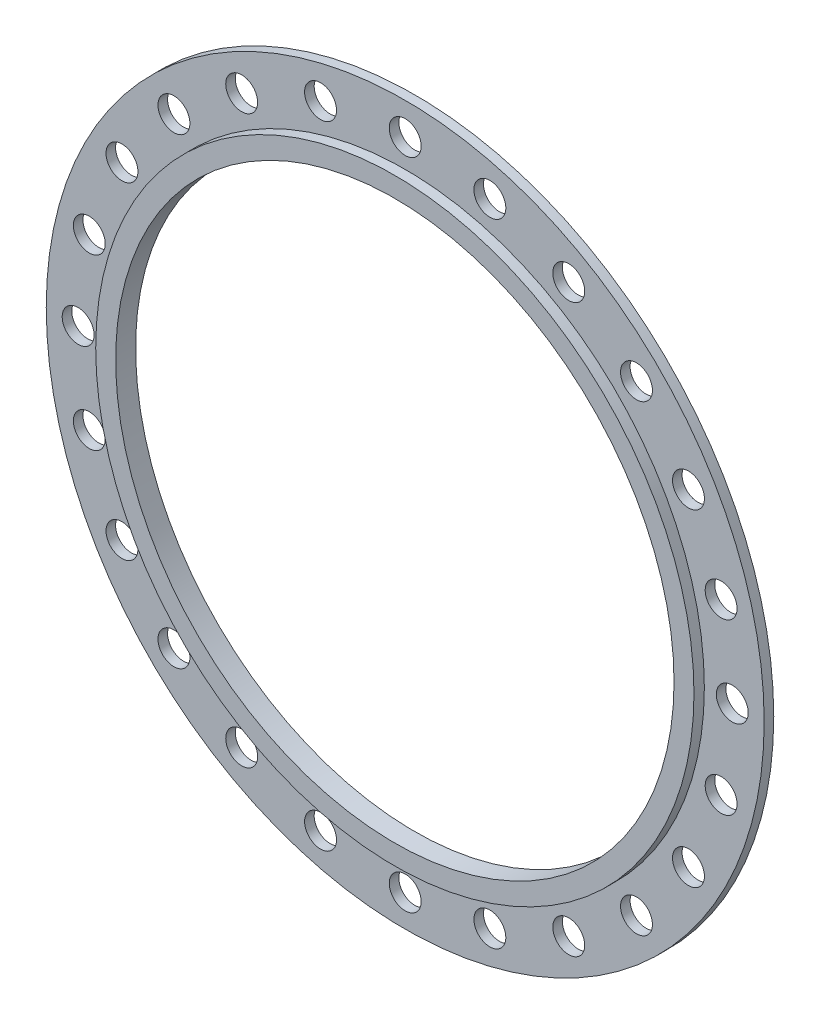
SolidWorks part; units mm, degrees
ref_plane "前视基准面" through (0, 0, 0) normal (0, 0, 1) x (1, 0, 0)
ref_plane "上视基准面" through (0, 0, 0) normal (0, 1, 0) x (1, 0, 0)
ref_plane "右视基准面" through (0, 0, 0) normal (1, 0, 0) x (0, 0, -1)
other "Configuration Table"
sketch "草图1" plane through (0, 0, 0) normal (0, 0, 1) x (1, 0, 0)
  circle A0 centre (0, 0) radius 450
  dimension "D1" = 900
extrude "凸台-拉伸1" add sketch "草图1" along normal blind 12 contours A0
sketch "草图2" plane through (0, 0, 12) normal (0, 0, 1) x (1, 0, 0)
  circle A0 centre (0, 0) radius 375
  dimension "D1" = 750
extrude "凸台-拉伸2" add sketch "草图2" along normal blind 13 contours A0
sketch "草图3" plane through (0, 0, 0) normal (0, 0, -1) x (-1, 0, 0)
  circle A0 centre (0, 0) radius 410 construction
  circle A1 centre (0, 410) radius 20
  circle A2 centre (106.1158, 396.0296) radius 20
  circle A3 centre (205, 355.0704) radius 20
  circle A4 centre (289.9138, 289.9138) radius 20
  circle A5 centre (355.0704, 205) radius 20
  circle A6 centre (396.0296, 106.1158) radius 20
  circle A7 centre (410, 0) radius 20
  circle A8 centre (396.0296, -106.1158) radius 20
  circle A9 centre (355.0704, -205) radius 20
  circle A10 centre (289.9138, -289.9138) radius 20
  circle A11 centre (205, -355.0704) radius 20
  circle A12 centre (106.1158, -396.0296) radius 20
  circle A13 centre (0, -410) radius 20
  circle A14 centre (-106.1158, -396.0296) radius 20
  circle A15 centre (-205, -355.0704) radius 20
  circle A16 centre (-289.9138, -289.9138) radius 20
  circle A17 centre (-355.0704, -205) radius 20
  circle A18 centre (-396.0296, -106.1158) radius 20
  circle A19 centre (-410, 0) radius 20
  circle A20 centre (-396.0296, 106.1158) radius 20
  circle A21 centre (-355.0704, 205) radius 20
  circle A22 centre (-289.9138, 289.9138) radius 20
  circle A23 centre (-205, 355.0704) radius 20
  circle A24 centre (-106.1158, 396.0296) radius 20
  dimension "D1" = 820
  dimension "D2" = 40
  dimension "D3" = 24
extrude "切除-拉伸2" cut sketch "草图3" against normal blind 314
sketch "草图4" plane through (0, 0, 25) normal (0, 0, 1) x (1, 0, 0)
  circle A0 centre (0, 0) radius 350
  dimension "D1" = 700
extrude "切除-拉伸3" cut sketch "草图4" against normal blind 314 contours A0
